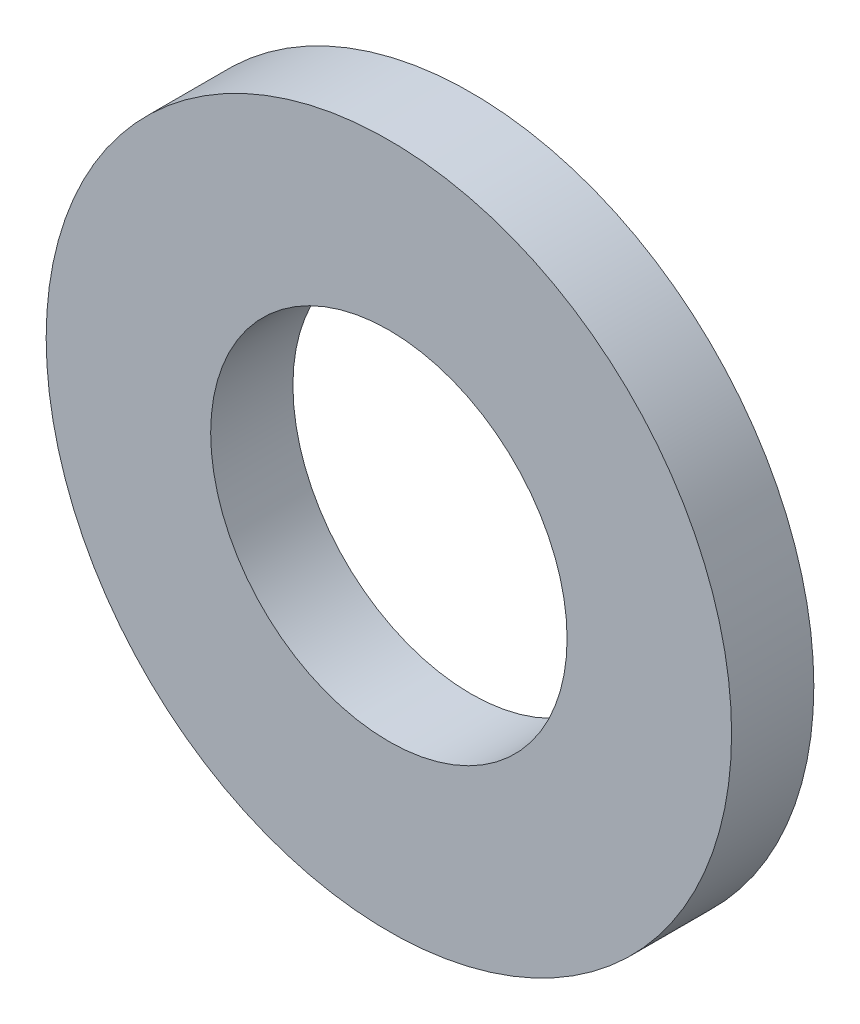
SolidWorks part; units mm, degrees
ref_plane "Front Plane" through (0, 0, 0) normal (0, 0, 1) x (1, 0, 0)
ref_plane "Top Plane" through (0, 0, 0) normal (0, 1, 0) x (1, 0, 0)
ref_plane "Right Plane" through (0, 0, 0) normal (1, 0, 0) x (0, 0, -1)
sketch "Sketch1" plane through (0, 0, 0) normal (0, 0, 1) x (1, 0, 0)
  circle A0 centre (0, 0) radius 12.5
  circle A1 centre (0, 0) radius 6.5
  dimension "D1" = 25
  dimension "D2" = 13
extrude "Boss-Extrude1" add sketch "Sketch1" along normal blind 3
